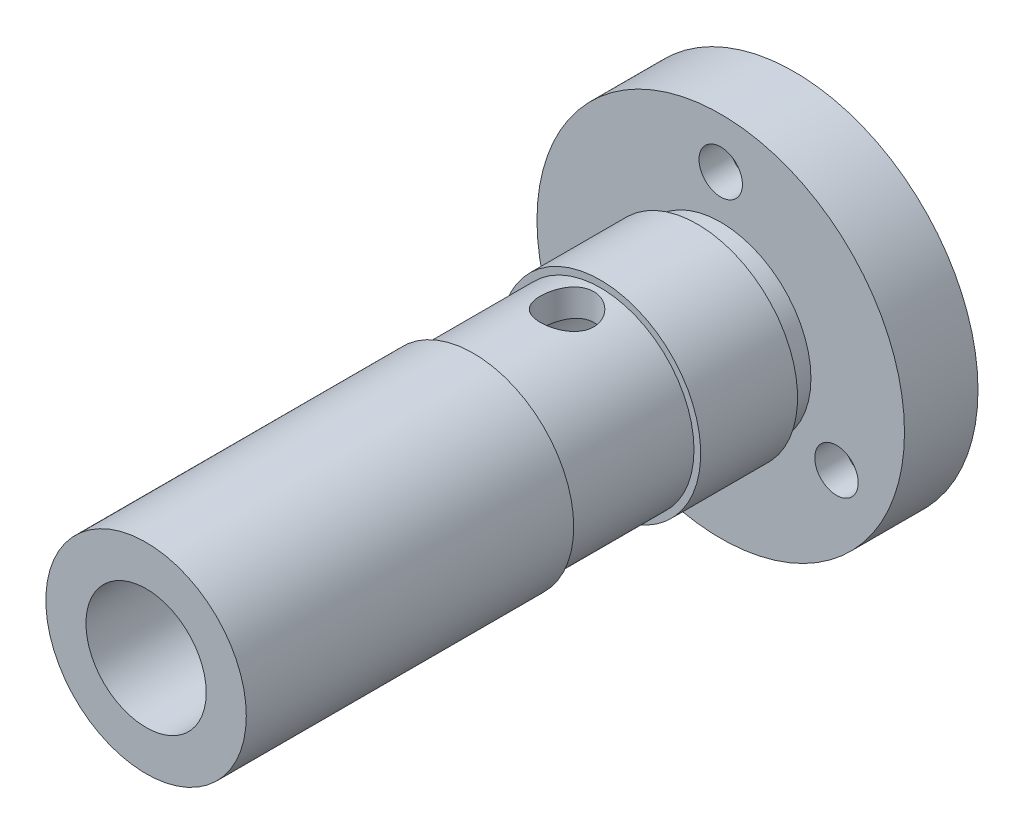
SolidWorks part; units mm, degrees
ref_plane "Front Plane" through (0, 0, 0) normal (0, 0, 1) x (1, 0, 0)
ref_plane "Top Plane" through (0, 0, 0) normal (0, 1, 0) x (1, 0, 0)
ref_plane "Right Plane" through (0, 0, 0) normal (1, 0, 0) x (0, 0, -1)
other "Configuration Table"
sketch "Sketch1" plane through (0, 0, 0) normal (0, 0, 1) x (1, 0, 0)
  circle A0 centre (0, 0) radius 27.5
  dimension "D1" = 55
extrude "Boss-Extrude1" add sketch "Sketch1" along normal blind 11
sketch "Sketch2" plane through (0, 0, 11) normal (0, 0, 1) x (1, 0, 0)
  circle A0 centre (0, 0) radius 13.5
  dimension "D1" = 27
extrude "Boss-Extrude2" add sketch "Sketch2" along normal blind 3.5
sketch "Sketch3" plane through (0, 0, 14.5) normal (0, 0, 1) x (1, 0, 0)
  circle A0 centre (0, 0) radius 15
  dimension "D1" = 30
extrude "Boss-Extrude3" add sketch "Sketch3" along normal blind 14.5
sketch "Sketch4" plane through (0, 0, 29) normal (0, 0, 1) x (1, 0, 0)
  circle A0 centre (0, 0) radius 14
  dimension "D1" = 28
extrude "Boss-Extrude4" add sketch "Sketch4" along normal blind 19
sketch "Sketch5" plane through (0, 0, 48) normal (0, 0, 1) x (1, 0, 0)
  circle A0 centre (0, 0) radius 15
  dimension "D1" = 30
extrude "Boss-Extrude5" add sketch "Sketch5" along normal blind 49
sketch "Sketch6" plane through (0, 0, 97) normal (0, 0, 1) x (1, 0, 0)
  circle A0 centre (0, 0) radius 9
  dimension "D1" = 18
extrude "Cut-Extrude1" cut sketch "Sketch6" against normal blind 52
sketch "Sketch7" plane through (0, 0, 45) normal (0, 0, 1) x (1, 0, 0)
  circle A0 centre (0, 0) radius 10
  dimension "D1" = 20
extrude "Cut-Extrude2" cut sketch "Sketch7" against normal blind 38
sketch "Sketch8" plane through (0, 0, 0) normal (0, 0, -1) x (-1, 0, 0)
  line L0 (0, 0) -> (0, 26.4793) construction
  circle A0 centre (0, 20) radius 5.5
  dimension "D2" = 11
  dimension "D1" = 20
extrude "Cut-Extrude3" cut sketch "Sketch8" against normal blind 6.5
sketch "Sketch9" plane through (0, 0, 6.5) normal (0, 0, -1) x (-1, 0, 0)
  circle A0 centre (0, 20) radius 3.25
  dimension "D1" = 6.5
extrude "Cut-Extrude4" cut sketch "Sketch9" against normal blind 6.5
pattern_circular "CirPattern1" count 3 over 360 about axis through (0, 0, 0) along (0, 0, 1) of "Cut-Extrude3", "Cut-Extrude4"
sketch "Sketch10" plane through (0, 0, 0) normal (0, 1, 0) x (1, 0, 0)
  circle A0 centre (0, -34) radius 4
  dimension "D1" = 8
  dimension "D2" = 34
extrude "Cut-Extrude5" cut sketch "Sketch10" against normal mid plane 53.5
